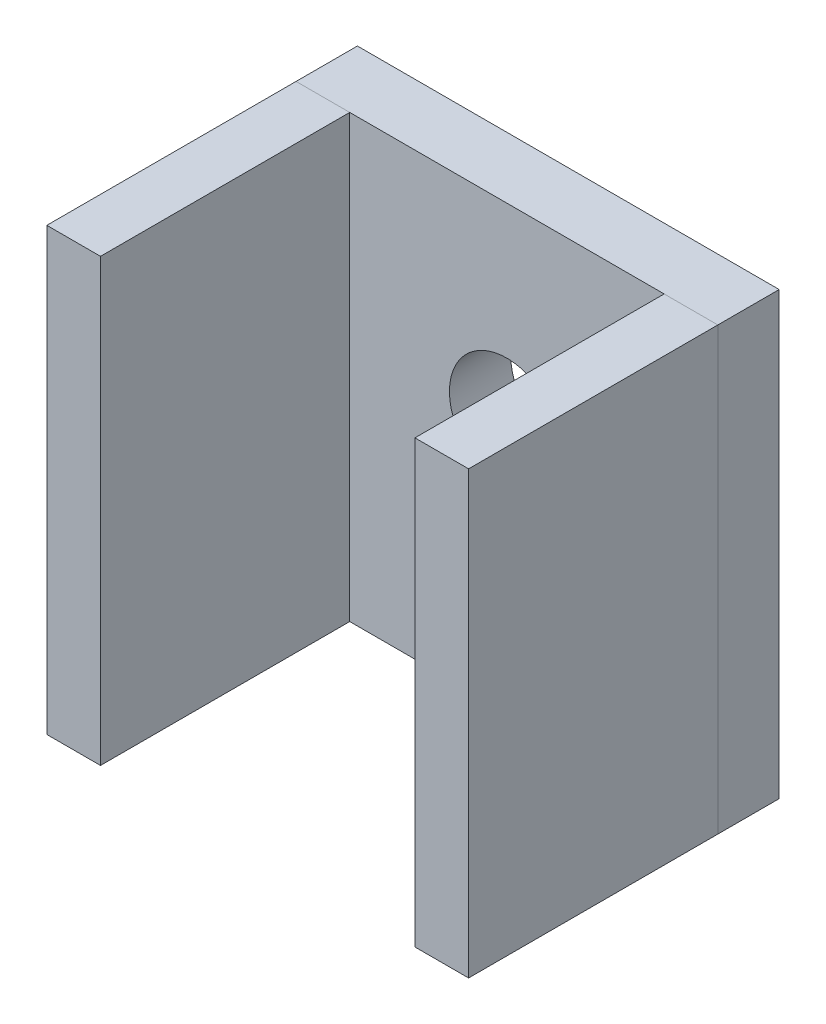
SolidWorks part; units mm, degrees
ref_plane "前视基准面" through (0, 0, 0) normal (0, 0, 1) x (1, 0, 0)
ref_plane "上视基准面" through (0, 0, 0) normal (0, 1, 0) x (1, 0, 0)
ref_plane "右视基准面" through (0, 0, 0) normal (1, 0, 0) x (0, 0, -1)
other "Configuration Table"
sketch "草图1" plane through (0, 0, 0) normal (0, 0, 1) x (1, 0, 0)
  line L1 (-55, -50) -> (55, -50)
  line L2 (-55, -50) -> (-55, 50)
  line L3 (-55, 50) -> (55, 50)
  line L4 (55, -50) -> (55, 50)
  line L5 (0, 50) -> (0, -50) construction
  line L6 (-55, 0) -> (55, 0) construction
  point P0 (0, 0)
  dimension "D1" = 110
  dimension "D2" = 100
extrude "凸台-拉伸1" add sketch "草图1" along normal blind 16
sketch "草图2" plane through (-55, 0, 0) normal (-1, 0, 0) x (0, 0, 1)
  line L0 (16, 50) -> (16, -65)
  line L1 (16, -65) -> (81, -65)
  line L6 (16, 50) -> (81, 50)
  line L7 (81, 50) -> (81, -65)
  dimension "D1" = 115
  dimension "D3" = 65
extrude "凸台-拉伸2" add sketch "草图2" against normal blind 14 separate body
mirror "镜向1" about plane through (0, 0, 0) normal (1, 0, 0) of bodies 107
sketch "草图3" plane through (0, 0, 0) normal (0, 0, -1) x (-1, 0, 0)
  circle A0 centre (0, 0) radius 15
  dimension "D1" = 30
extrude "切除-拉伸1" cut sketch "草图3" against normal up to next (16 mm away)
sketch "草图4" plane through (0, -50, 0) normal (0, -1, 0) x (1, 0, 0)
  line L1 (-55, 16) -> (55, 16)
  line L2 (-55, 16) -> (-55, 0)
  line L3 (-55, 0) -> (55, 0)
  line L4 (55, 16) -> (55, 0)
extrude "凸台-拉伸3" add sketch "草图4" along normal up to surface (15 mm away) up to face at (-48, -65, 48.5)
